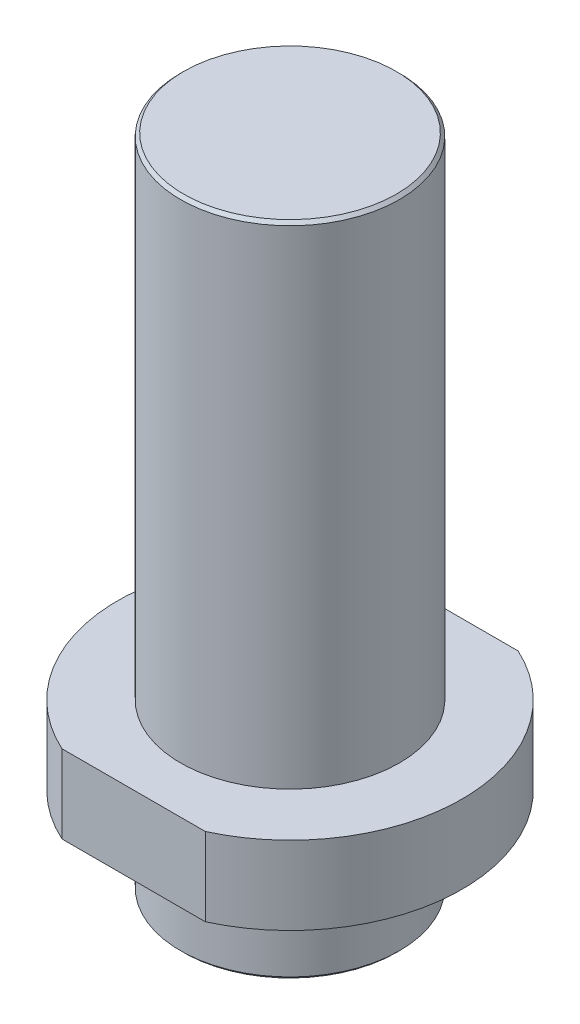
SolidWorks part; units mm, degrees
material "45"
ref_plane "Front Plane" through (0, 0, 0) normal (0, 0, 1) x (1, 0, 0)
ref_plane "Top Plane" through (0, 0, 0) normal (0, 1, 0) x (1, 0, 0)
ref_plane "Right Plane" through (0, 0, 0) normal (1, 0, 0) x (0, 0, -1)
sketch "Sketch1" plane through (0, 0, 0) normal (0, 0, 1) x (1, 0, 0)
  line L0 (0, 0) -> (-34, 0)
  line L1 (-35, 1) -> (-35, 28)
  line L2 (-35, 28) -> (-55, 28)
  line L3 (-55, 28) -> (-55, 53)
  line L4 (-55, 53) -> (-35, 53)
  line L5 (-35, 53) -> (-35, 209)
  line L6 (-34, 210) -> (0, 210)
  line L7 (0, 210) -> (0, 0)
  line L8 (-35, 209) -> (-34, 210)
  line L9 (-34, 0) -> (-35, 1)
  point P1 (-35, 0)
  point P8 (-35, 210)
  dimension "D1" = 210
  dimension "D2" = 35
  dimension "D3" = 28
  dimension "D4" = 25
  dimension "D5" = 55
revolve "Revolve1" add sketch "Sketch1" angle 360 about L7
sketch "Sketch2" plane through (0, 53, 0) normal (0, 1, 0) x (1, 0, 0)
  line L0 (-22.9129, 50) -> (22.9129, 50)
  line L1 (-22.9129, -50) -> (22.9129, -50)
  circle A0 centre (0, 0) radius 55 construction
  arc A1 (-22.9129, -50) -> (22.9129, -50) centre (0, 0) ccw
  arc A2 (22.9129, 50) -> (-22.9129, 50) centre (0, 0) ccw
  dimension "D1" = 100
  dimension "D2" = 50
extrude "Cut-Extrude1" cut sketch "Sketch2" against normal through all
